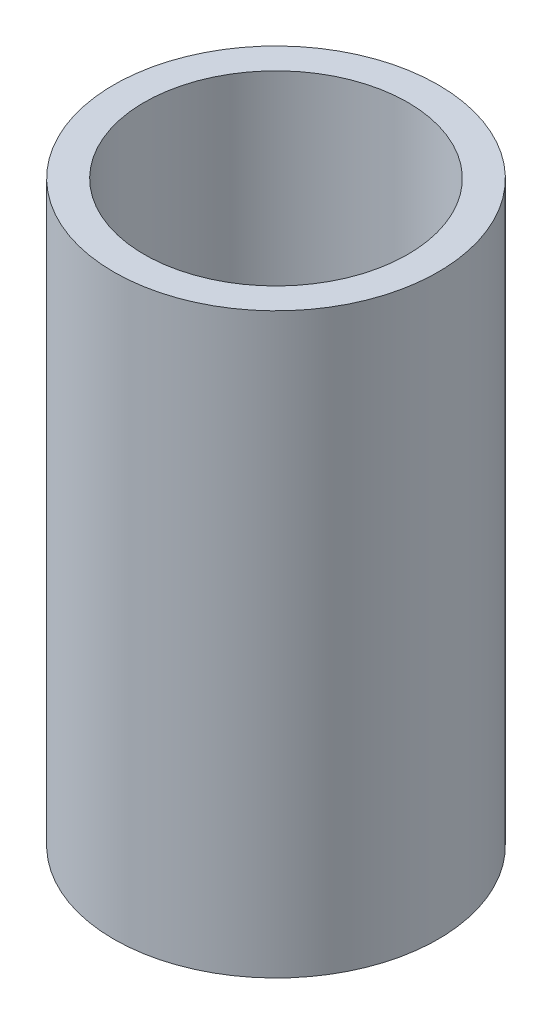
SolidWorks part; units mm, degrees
material "Q235B"
ref_plane "Front Plane" through (0, 0, 0) normal (0, 0, 1) x (1, 0, 0)
ref_plane "Top Plane" through (0, 0, 0) normal (0, 1, 0) x (1, 0, 0)
ref_plane "Right Plane" through (0, 0, 0) normal (1, 0, 0) x (0, 0, -1)
sketch "Sketch1" plane through (0, 0, 0) normal (0, 1, 0) x (1, 0, 0)
  circle A0 centre (0, 0) radius 16
  circle A1 centre (0, 0) radius 13
  dimension "D1" = 32
  dimension "D2" = 26
extrude "Boss-Extrude1" add sketch "Sketch1" along normal blind 57
chamfer "Chamfer2" [suppressed] distance 0.5 angle 45
